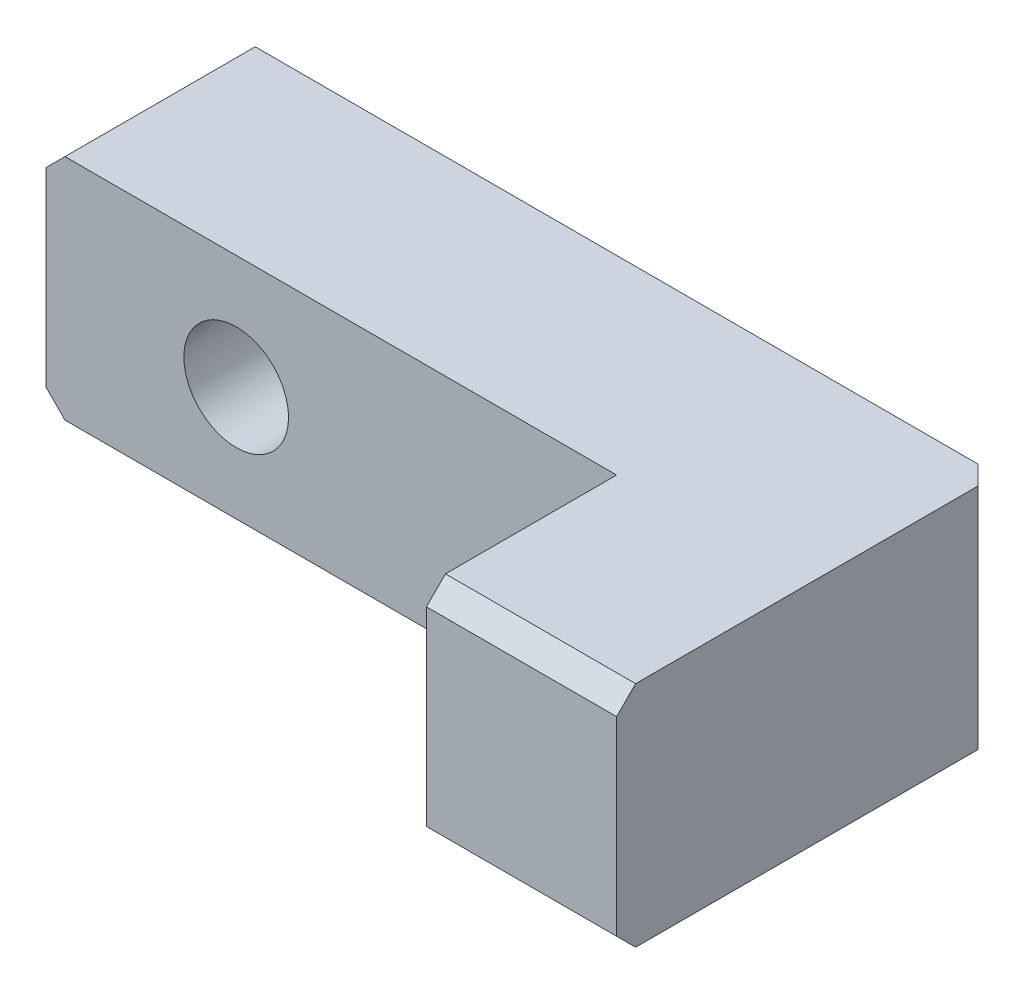
from build123d import *

# Parameters (mm, degrees)
SKETCH_1_W                = 40
SKETCH_1_H                = 20
EXTRUDE_1_DEPTH           = 6
SKETCH_2_W                = 30
SKETCH_2_H                = 10
CUT_EXTRUDE_1_DEPTH       = 12
HOLE_WIZARD_1_D           = 5.5
HOLE_WIZARD_1_CBORE_D     = 10
HOLE_WIZARD_1_CBORE_DEPTH = 5.7
CHAMFER_1_SIZE            = 1


with BuildPart() as part:
    # 草图1 → 凸台-拉伸1 (new, symmetric)
    with BuildSketch(Plane(origin=(0, 0, 0), x_dir=(1, 0, 0), z_dir=(0, 1, 0))):
        Rectangle(SKETCH_1_W, SKETCH_1_H)
    extrude(amount=EXTRUDE_1_DEPTH, both=True)

    # 草图2 → 切除-拉伸1 (cut)
    with BuildSketch(Plane(origin=(0, 6, 0), x_dir=(1, 0, 0), z_dir=(0, 1, 0))):
        with Locations((-5, -5)):
            Rectangle(SKETCH_2_W, SKETCH_2_H)
    extrude(amount=-CUT_EXTRUDE_1_DEPTH, mode=Mode.SUBTRACT)

    # 打孔尺寸(%根据)内六角圆柱头螺钉的类型1 (through all)
    with Locations(Plane(origin=(0, 0, -10), x_dir=(-1, 0, 0), z_dir=(0, 0, -1))):
        with Locations((10, 0)):
            CounterBoreHole(HOLE_WIZARD_1_D / 2, HOLE_WIZARD_1_CBORE_D / 2, HOLE_WIZARD_1_CBORE_DEPTH)

    # 倒角1
    chamfer_1_edges = [part.edges().sort_by_distance(p)[0] for p in [
        (-20, 6, -5),
        (15, -6, 10),
        (15, 6, 10),
        (-20, -6, -5),
        (20, 0, -10),
    ]]
    chamfer(chamfer_1_edges, length=CHAMFER_1_SIZE)


solid = part.part
